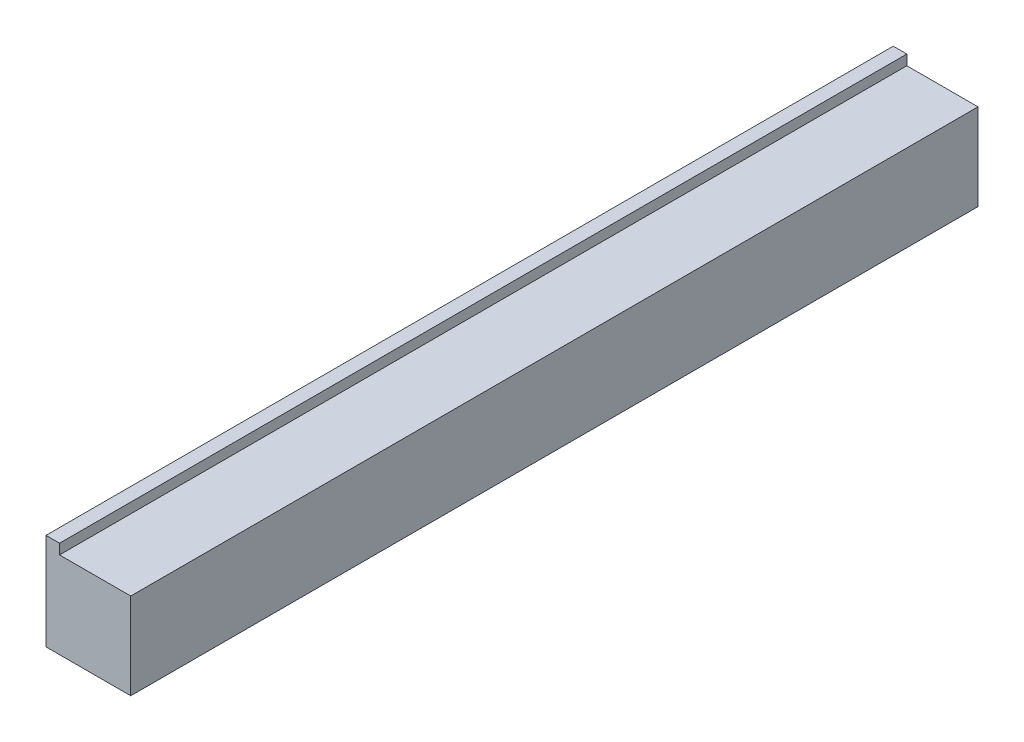
SolidWorks part; units mm, degrees
ref_plane "前视基准面" through (0, 0, 0) normal (0, 0, 1) x (1, 0, 0)
ref_plane "上视基准面" through (0, 0, 0) normal (0, 1, 0) x (1, 0, 0)
ref_plane "右视基准面" through (0, 0, 0) normal (1, 0, 0) x (0, 0, -1)
sketch "草图1" plane through (0, 0, 0) normal (0, 0, 1) x (1, 0, 0)
  line L0 (-10, -12.5) -> (-14, -12.5)
  line L1 (-10, -10.2831) -> (-10, -14.5) construction
  line L2 (-14, -12.5) -> (-14, -41)
  line L3 (-14, -41) -> (11, -41)
  line L4 (11, -41) -> (11, -15.5)
  line L5 (11, -15.5) -> (-10, -15.5)
  line L6 (-10, -15.5) -> (-10, -12.5)
  dimension "D1" = 25.5
  dimension "D2" = 3
  dimension "D3" = 4
  dimension "D4" = 25
  dimension "D5" = 15.5
extrude "凸台-拉伸1" add sketch "草图1" against normal blind 250
